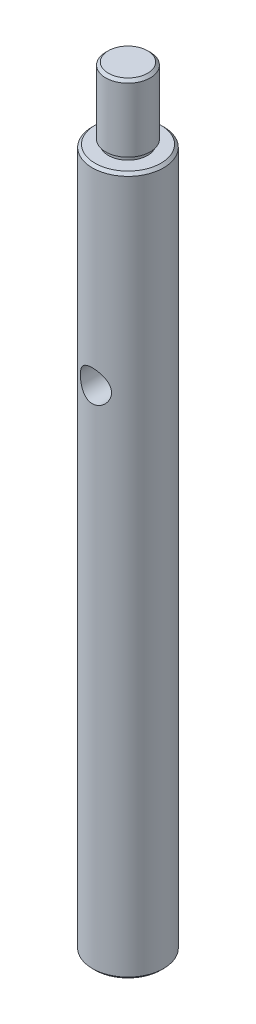
from build123d import *

# Parameters (mm, degrees)
SKETCH1_R             = 4
BOSS_EXTRUDE1_DEPTH   = 78.5
SKETCH2_R             = 2.5
BOSS_EXTRUDE2_DEPTH   = 8
CHAMFER1_SIZE         = 0.3
M4_TAPPED_HOLE1_D     = 3.3
M4_TAPPED_HOLE1_DEPTH = 10.1
M4_TAPPED_HOLE1_TIP   = 0.991420021
SKETCH6_R             = 1.75
CUT_EXTRUDE1_DEPTH    = 5
SKETCH7_W             = 0.3
SKETCH7_H             = 0.5


with BuildPart() as part:
    # Sketch1 → Boss-Extrude1 (new body)
    with BuildSketch(Plane(origin=(0, 0, 0), x_dir=(1, 0, 0), z_dir=(0, 1, 0))):
        with Locations(Location((0, 0, 0), (0, 0, 270))):
            Circle(SKETCH1_R)
    extrude(amount=BOSS_EXTRUDE1_DEPTH)

    # Sketch2 → Boss-Extrude2 (add)
    with BuildSketch(Plane(origin=(0, 78.5, 0), x_dir=(1, 0, 0), z_dir=(0, 1, 0))):
        with Locations(Location((0, 0, 0), (0, 0, 270))):
            Circle(SKETCH2_R)
    extrude(amount=BOSS_EXTRUDE2_DEPTH)

    # Chamfer1
    chamfer1_edges = [part.edges().sort_by_distance(p)[0] for p in [
        (0, 0, -4),
        (0, 78.5, -4),
        (0, 86.5, -2.5),
    ]]
    chamfer(chamfer1_edges, length=CHAMFER1_SIZE)

    # M4 Tapped Hole1
    with Locations(Plane(origin=(0, 0, 0), x_dir=(-1, 0, 0), z_dir=(0, -1, 0))):
        with Locations((0, 0)):
            Hole(M4_TAPPED_HOLE1_D / 2, depth=M4_TAPPED_HOLE1_DEPTH)
            with Locations((0, 0, -(M4_TAPPED_HOLE1_DEPTH + M4_TAPPED_HOLE1_TIP / 2))):  # 118° drill point
                Cone(0, M4_TAPPED_HOLE1_D / 2, M4_TAPPED_HOLE1_TIP, mode=Mode.SUBTRACT)

    # Sketch6 → Cut-Extrude1 (cut, symmetric)
    with BuildSketch(Plane.XY):
        with Locations(Location((0, 57, 0), (0, 0, 90))):
            Circle(SKETCH6_R)
    extrude(amount=CUT_EXTRUDE1_DEPTH, both=True, mode=Mode.SUBTRACT)

    # Sketch7 → Cut-Revolve1 (revolve, cut)
    with BuildSketch(Plane.XY, mode=Mode.PRIVATE) as cut_revolve1_sk:
        with Locations((2.35, 78.75)):
            Rectangle(SKETCH7_W, SKETCH7_H)
    revolve(cut_revolve1_sk.sketch.rotate(Axis((0, 0, 0), (0, 1, 0)), 90), axis=Axis((0, 0, 0), (0, 1, 0)), mode=Mode.SUBTRACT)


solid = part.part
